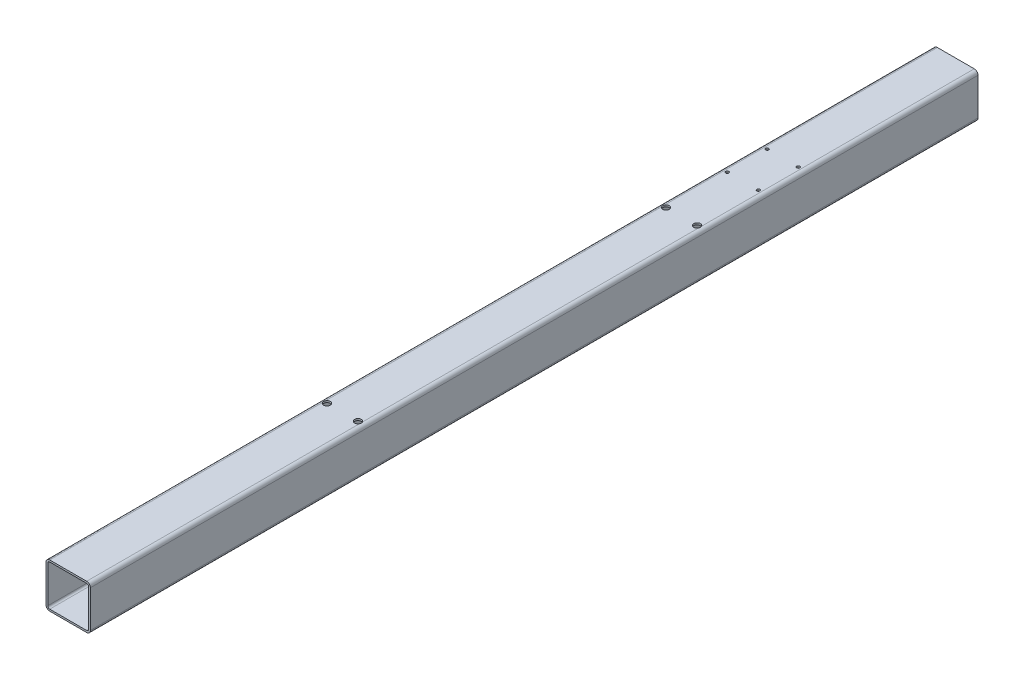
SolidWorks part; units mm, degrees
material "1023 碳钢板 (SS)"
ref_plane "Front Plane" through (0, 0, 0) normal (0, 0, 1) x (1, 0, 0)
ref_plane "Top Plane" through (0, 0, 0) normal (0, 1, 0) x (1, 0, 0)
ref_plane "Right Plane" through (0, 0, 0) normal (1, 0, 0) x (0, 0, -1)
sketch "Sketch1" plane through (0, 0, 0) normal (0, 0, 1) x (1, 0, 0)
  line L1 (50, 50) -> (-50, 50)
  line L2 (50, 50) -> (50, -50)
  line L3 (50, -50) -> (-50, -50)
  line L4 (-50, 50) -> (-50, -50)
  line L5 (50, 50) -> (-50, -50) construction
  line L6 (50, -50) -> (-50, 50) construction
  point P0 (0, 0)
  dimension "D1" = 100
  dimension "D2" = 100
extrude "Boss-Extrude1" add sketch "Sketch1" along normal blind 2000
fillet "Fillet1" radius 8.4 4 edges at (50, -50, 1000) (-50, -50, 1000) (-50, 50, 1000) (50, 50, 1000)
shell "Shell1" thickness 4
sketch "Sketch2" plane through (0, 50, 0) normal (0, 1, 0) x (1, 0, 0)
  line L1 (50, 0) -> (50, -2000) construction
  line L2 (41.6, 0) -> (-41.6, 0) construction
  circle A0 centre (35, -618) radius 7.5
  circle A1 centre (-35, -618) radius 7.5
  circle A2 centre (35, -1382) radius 7.5
  circle A3 centre (-35, -1382) radius 7.5
  circle A4 centre (-35, -390) radius 3
  circle A5 centre (35, -390) radius 3
  circle A6 centre (35, -480) radius 3
  circle A7 centre (-35, -480) radius 3
  dimension "D9" = 6
  dimension "D10" = 15
  dimension "D1" = 70
  dimension "D2" = 35
  dimension "D3" = 70
  dimension "D4" = 15
  dimension "D5" = 90
  dimension "D6" = 764
  dimension "D7" = 390
  dimension "D8" = 618
hole_wizard "M8 Tapped Hole1" positions "Sketch5" profile "Sketch6" tap size "M8" standard "ISO"
sketch "Sketch5" plane through (0, 50, 0) normal (0, 1, 0) x (1, 0, 0)
  point P0 (-35, -390)
  point P3 (35, -390)
  point P6 (35, -480)
  point P9 (-35, -480)
sketch "Sketch6" plane through (-35, 50, 390) normal (1, 0, 0) x (0, 0, 1)
  line L0 (0, 0) -> (0, 21.7929)
  line L1 (0, 21.7929) -> (3.4, 19.75)
  line L2 (3.4, 19.75) -> (3.4, 0)
  line L5 (3.4, 0) -> (0, 0)
  line L10 (0, 21.7929) -> (-3.4, 19.75) construction
  line L11 (0, -6.35) -> (0, 107.95) construction
  dimension "螺纹孔钻头直径" = 6.8
  dimension "螺纹孔钻头深度" = 19.75
  dimension "导头角度" = 118
cosmetic thread "Hole Thread Line 5" parameters "D1"=16, "D2"=8
cosmetic thread "Hole Thread Line 6" parameters "D1"=16, "D2"=8
cosmetic thread "Hole Thread Line 7" parameters "D1"=16, "D2"=8
cosmetic thread "Hole Thread Line 8" parameters "D1"=16, "D2"=8
extrude "Cut-Extrude1" cut sketch "Sketch2" against normal blind 10
